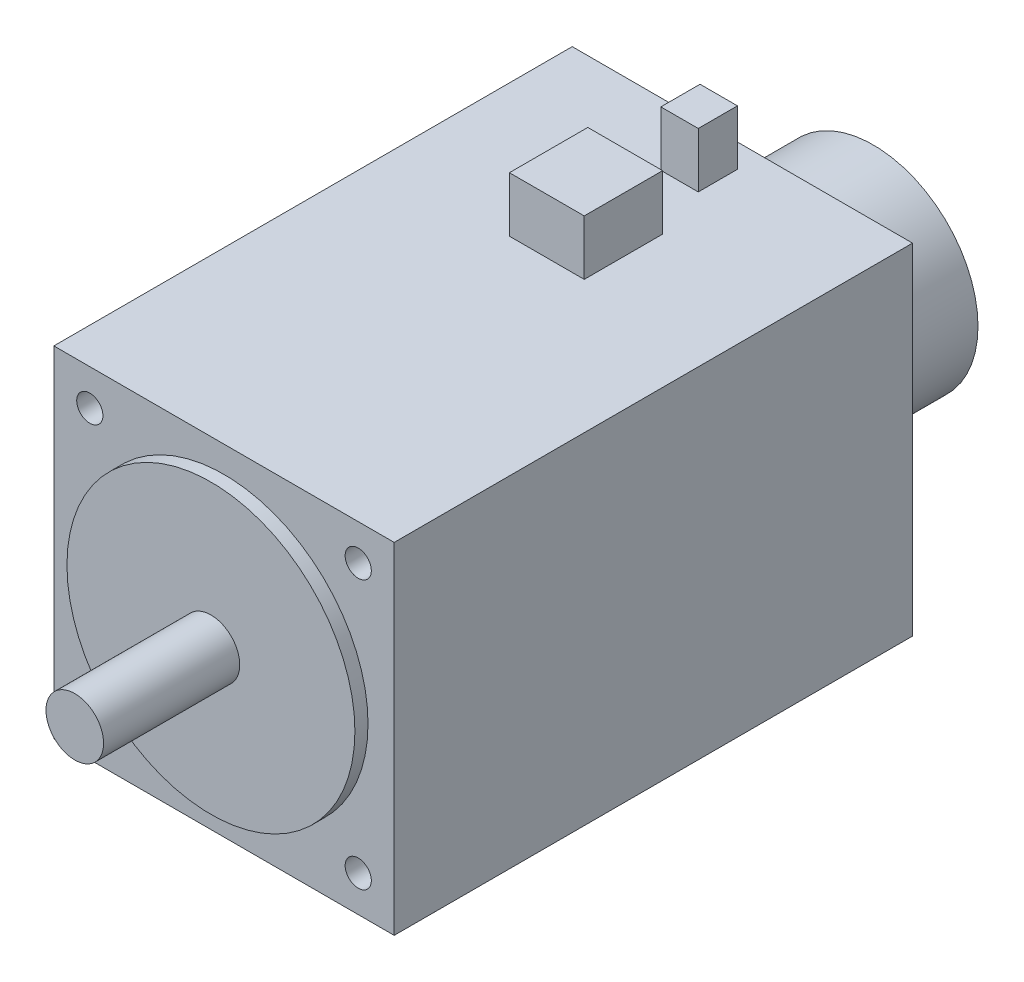
SolidWorks part; units mm, degrees
ref_plane "前视基准面" through (0, 0, 0) normal (0, 0, 1) x (1, 0, 0)
ref_plane "上视基准面" through (0, 0, 0) normal (0, 1, 0) x (1, 0, 0)
ref_plane "右视基准面" through (0, 0, 0) normal (1, 0, 0) x (0, 0, -1)
sketch "草图1" plane through (0, 0, 0) normal (0, 0, 1) x (1, 0, 0)
  line L0 (65, -65) -> (-65, 65) construction
  line L1 (-65, 65) -> (65, 65)
  line L2 (-65, 65) -> (-65, -65)
  line L3 (-65, -65) -> (65, -65)
  line L4 (65, 65) -> (65, -65)
  line L5 (0, 0) -> (0, 89.419) construction
  line L6 (0, 0) -> (106.8518, 0) construction
  circle A0 centre (-51.2652, 51.2652) radius 5
  circle A1 centre (51.2652, 51.2652) radius 5
  circle A2 centre (-51.2652, -51.2652) radius 5
  circle A3 centre (51.2652, -51.2652) radius 5
  dimension "D1" = 130
  dimension "D2" = 10
  dimension "D3" = 145
extrude "凸台-拉伸1" add sketch "草图1" along normal mid plane 198
sketch "草图2" plane through (0, 0, 99) normal (0, 0, 1) x (1, 0, 0)
  circle A0 centre (0, 0) radius 55
  dimension "D1" = 110
extrude "凸台-拉伸2" add sketch "草图2" along normal blind 5
sketch "草图3" plane through (0, 0, 104) normal (0, 0, 1) x (1, 0, 0)
  circle A0 centre (0, 0) radius 11
  dimension "D1" = 22
extrude "凸台-拉伸3" add sketch "草图3" along normal blind 52
sketch "草图5" plane through (0, 0, 0) normal (0, 1, 0) x (1, 0, 0)
  line L1 (14.2922, 24.297) -> (-14.2922, 24.297)
  line L2 (14.2922, 24.297) -> (14.2922, 54.2425)
  line L3 (14.2922, 54.2425) -> (-14.2922, 54.2425)
  line L4 (-14.2922, 24.297) -> (-14.2922, 54.2425)
  line L5 (14.2922, 24.297) -> (-14.2922, 54.2425) construction
  line L6 (14.2922, 54.2425) -> (-14.2922, 24.297) construction
  line L7 (7.1461, 75.0002) -> (-7.1461, 75.0002)
  line L8 (7.1461, 75.0002) -> (7.1461, 89.9729)
  line L9 (7.1461, 89.9729) -> (-7.1461, 89.9729)
  line L10 (-7.1461, 75.0002) -> (-7.1461, 89.9729)
  line L11 (7.1461, 75.0002) -> (-7.1461, 89.9729) construction
  line L12 (7.1461, 89.9729) -> (-7.1461, 75.0002) construction
  point P0 (0, 39.2698)
  point P5 (0, 82.4865)
extrude "凸台-拉伸4" add sketch "草图5" along normal blind 86
sketch "草图6" plane through (0, 0, -99) normal (0, 0, -1) x (-1, 0, 0)
  circle A0 centre (0, 0) radius 40
  dimension "D1" = 80
extrude "凸台-拉伸5" add sketch "草图6" along normal blind 50
